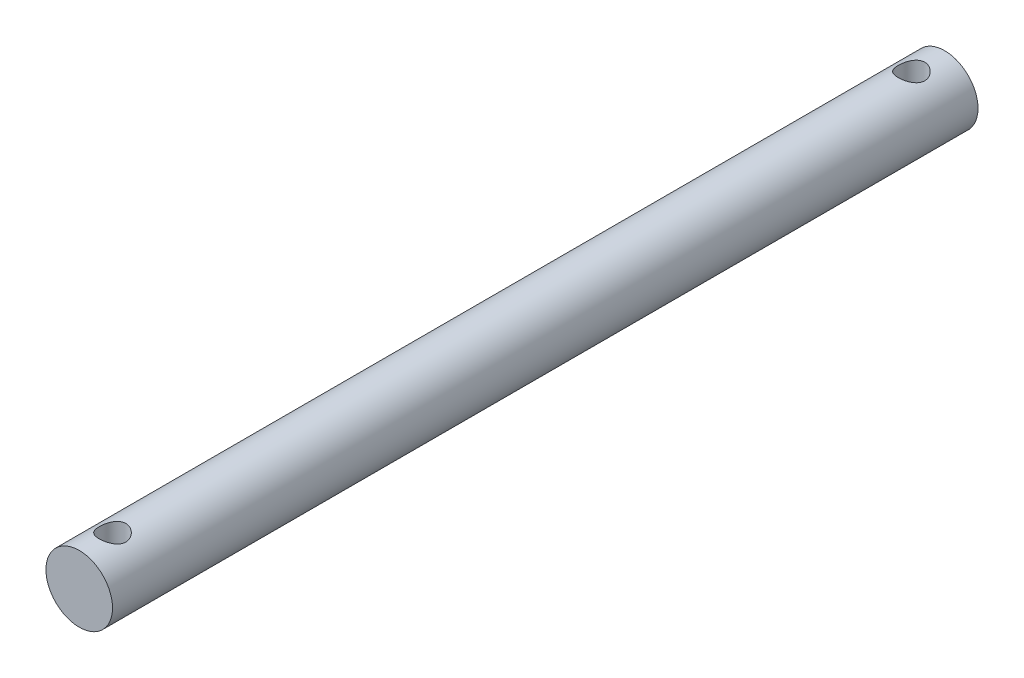
SolidWorks part; units mm, degrees
ref_plane "前视基准面" through (0, 0, 0) normal (0, 0, 1) x (1, 0, 0)
ref_plane "上视基准面" through (0, 0, 0) normal (0, 1, 0) x (1, 0, 0)
ref_plane "右视基准面" through (0, 0, 0) normal (1, 0, 0) x (0, 0, -1)
sketch "草图1" plane through (0, 0, 0) normal (0, 0, 1) x (1, 0, 0)
  circle A0 centre (0, 0) radius 5
  dimension "D1" = 10
extrude "凸台-拉伸1" add sketch "草图1" along normal mid plane 130
ref_plane "基准面1" through (0, 5, 0) normal (0, 1, 0) x (1, 0, 0)
sketch "草图2" plane through (0, 5, 0) normal (0, 1, 0) x (1, 0, 0)
  line L0 (0, -5.5) -> (0, 5.5) construction
  line L1 (-5.5, 0) -> (5.5, 0) construction
  circle A0 centre (0, -60) radius 2
  circle A1 centre (0, 60) radius 2
  dimension "D1" = 4
  dimension "D2" = 60
extrude "切除-拉伸1" cut sketch "草图2" against normal blind 10
